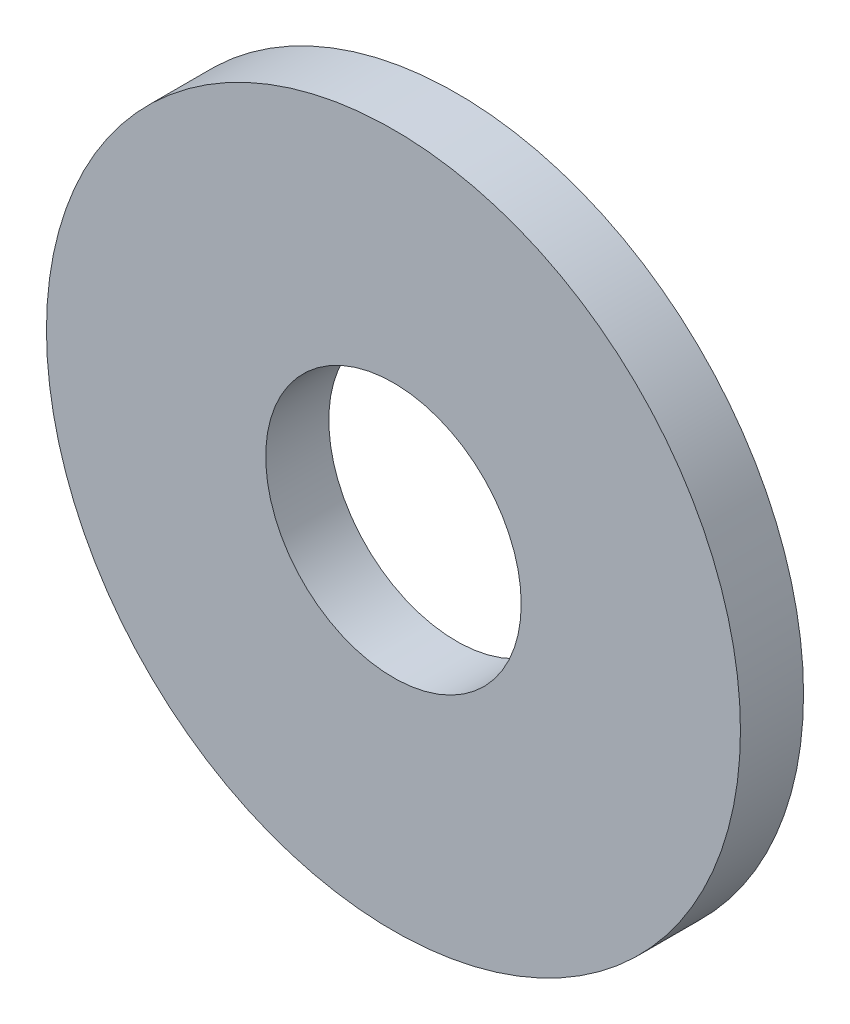
SolidWorks part; units mm, degrees
ref_plane "前视基准面" through (0, 0, 0) normal (0, 0, 1) x (1, 0, 0)
ref_plane "上视基准面" through (0, 0, 0) normal (0, 1, 0) x (1, 0, 0)
ref_plane "右视基准面" through (0, 0, 0) normal (1, 0, 0) x (0, 0, -1)
other "Configuration Table"
sketch "草图1" plane through (0, 0, 0) normal (0, 0, 1) x (1, 0, 0)
  circle A0 centre (0, 0) radius 22
  circle A1 centre (0, 0) radius 8.1
  point P0 (0, 0)
  dimension "D1" = 16.2
  dimension "D2" = 44
extrude "凸台-拉伸1" add sketch "草图1" against normal mid plane 4
